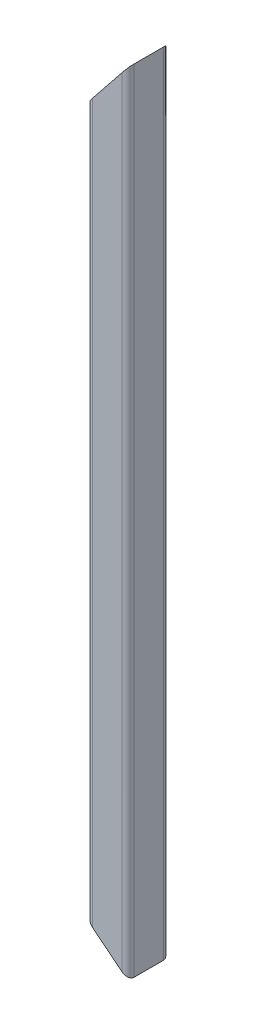
SolidWorks part; units mm, degrees
material "Q235B"
ref_plane "Front Plane" through (0, 0, 0) normal (0, 0, 1) x (1, 0, 0)
ref_plane "Top Plane" through (0, 0, 0) normal (0, 1, 0) x (1, 0, 0)
ref_plane "Right Plane" through (0, 0, 0) normal (1, 0, 0) x (0, 0, -1)
sketch "18 (ProfileFeature) (+7 more in 7 files) Sketch1" plane through (0, 0, 0) normal (0, 0, 1) x (1, 0, 0)
  line L0 (0, 0) -> (0, 1340)
  dimension "D1" = 1340
other "19 (WeldMemberFeat) (+4 more in 5 files) Cold-formed hollow square steel (GB/T 6728-2002) 70×70×5(1)"
ref_plane "Plane1" through (0, 0, 0) normal (0, 1, 0) x (-1, 0, 0)
sketch "Sketch1" plane through (0, 0, 0) normal (0, 1, 0) x (-1, 0, 0)
  line L0 (-25, -30) -> (25, -30)
  line L1 (-30, -25) -> (-30, 25)
  line L2 (25, 30) -> (-25, 30)
  line L3 (30, 25) -> (30, -25)
  line L4 (-25, -35) -> (25, -35)
  line L5 (-35, -25) -> (-35, 25)
  line L6 (25, 35) -> (-25, 35)
  line L7 (35, 25) -> (35, -25)
  arc A0 (35, 25) -> (25, 35) centre (25, 25) ccw
  arc A1 (25, -35) -> (35, -25) centre (25, -25) ccw
  arc A2 (-35, -25) -> (-25, -35) centre (-25, -25) ccw
  arc A3 (-25, 35) -> (-35, 25) centre (-25, 25) ccw
  arc A4 (-25, 30) -> (-30, 25) centre (-25, 25) ccw
  arc A5 (30, 25) -> (25, 30) centre (25, 25) ccw
  arc A6 (25, -30) -> (30, -25) centre (25, -25) ccw
  arc A7 (-30, -25) -> (-25, -30) centre (-25, -25) ccw
  point P0 (-35, 0)
  point P1 (35, 0)
  point P2 (0, 35)
  point P3 (0, -35)
  point P4 (0, 0)
  point P5 (-35, -35)
  point P6 (35, -35)
  point P7 (35, 35)
  point P8 (-35, 35)
  point P33 (0, 0)
  dimension "D1" = 10
  dimension "D2" = 70
  dimension "D3" = 5
sketch "Sketch2" plane through (0, 0, 35) normal (0, 0, 1) x (1, 0, 0)
  line L0 (35, 1340) -> (-35, 1252.5)
  line L1 (-35, 1340) -> (-35, 0) construction
  line L2 (-35, 1252.5) -> (-35, 1340)
  line L3 (-35, 1340) -> (35, 1340)
  line L4 (-35, 56) -> (35, 0)
  line L5 (35, 0) -> (-35, 0)
  line L6 (-35, 0) -> (-35, 56)
  dimension "D1" = 87.5
  dimension "D2" = 90
extrude "Cut-Extrude1" cut sketch "Sketch2" against normal through all both and the other way through all
